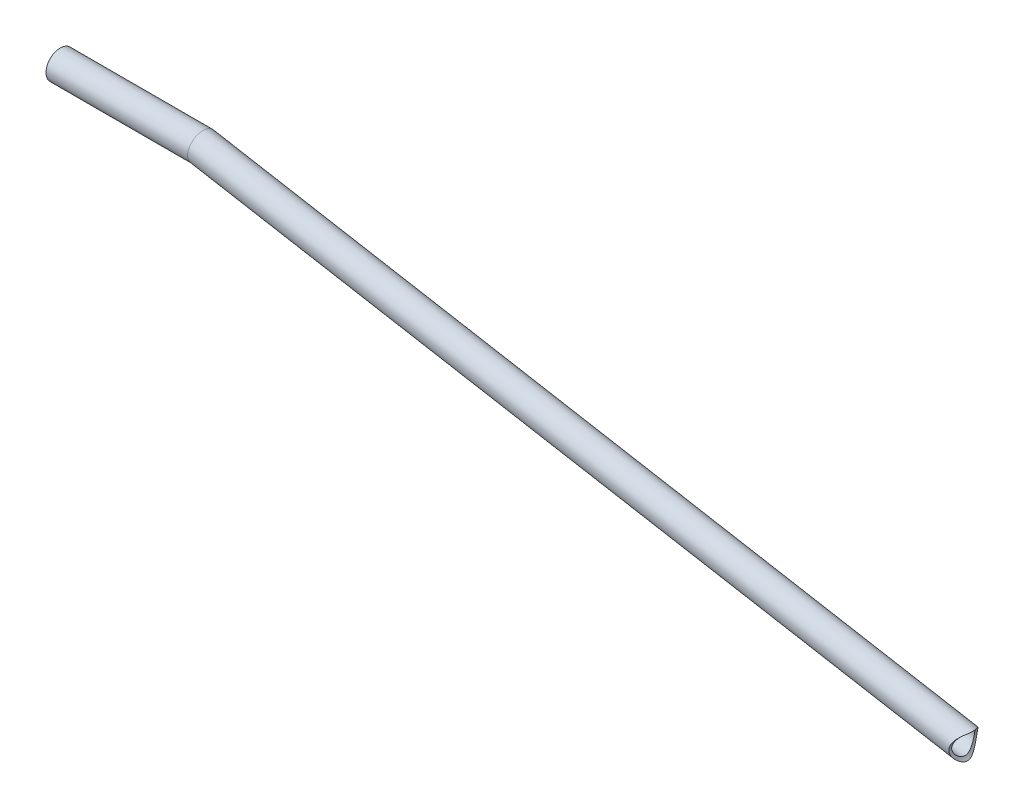
from build123d import *

# Parameters (mm, degrees)
SWEEP_THIN_1_PROFILE_R   = 10
SWEEP_THIN_1_PROFILE_R_2 = 8
CUT_EXTRUDE1_DEPTH       = 661.336346115
CUT_EXTRUDE1_DEPTH_BACK  = 661.336346115
SKETCH12_R               = 12.5


with BuildPart() as part:
    # Sweep-thin 1: sweep along a path in Sketch1
    with BuildLine(Plane.XY) as sweep_thin_1_path:
        Line((0, 0), (-551.248592867, 97.2))
        Line((-551.248592867, 97.2), (-651.5, 97.2))
    # Sweep-thin 1 profile (on start of the path) → Sweep-thin 1 (sweep)
    with BuildSketch(Plane(origin=(0, 0, 0), x_dir=(-0.1736481776669304, -0.9848077530122081, 0), z_dir=(-0.9848077530122081, 0.1736481776669304, 0))):
        Circle(SWEEP_THIN_1_PROFILE_R)
        Circle(SWEEP_THIN_1_PROFILE_R_2, mode=Mode.SUBTRACT)
    sweep(path=sweep_thin_1_path.line, transition=Transition.RIGHT)

    # Sketch12 → Cut-Extrude1 (cut, two sides: drawn at the far end of the back side and taken through both)
    with BuildSketch(Plane.XY.offset(-CUT_EXTRUDE1_DEPTH_BACK)):
        Circle(SKETCH12_R)
    extrude(amount=CUT_EXTRUDE1_DEPTH + CUT_EXTRUDE1_DEPTH_BACK, mode=Mode.SUBTRACT)


solid = part.part
